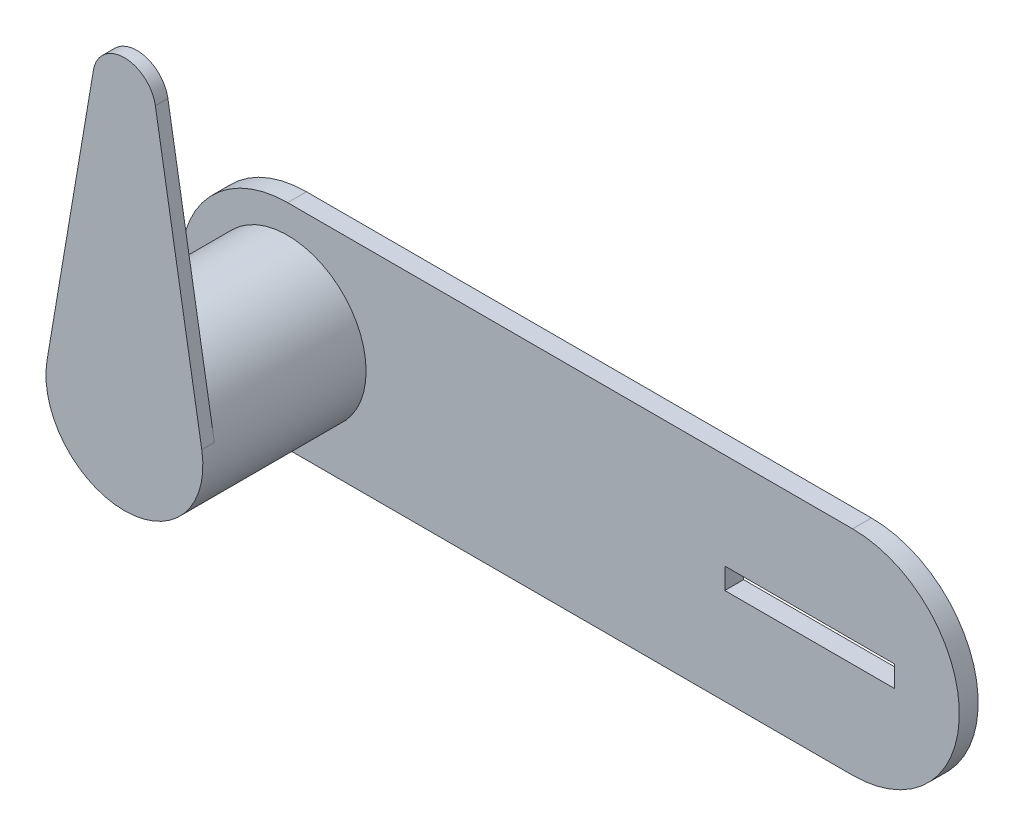
from build123d import *

# Parameters (mm, degrees)
EXTRUDE_1_DEPTH     = 3
SKETCH_2_W          = 27.052742461
SKETCH_2_H          = 3.381592808
CUT_EXTRUDE_1_DEPTH = 3
SKETCH_3_R          = 12.5
EXTRUDE_2_DEPTH     = 24
EXTRUDE_3_DEPTH     = 2


with BuildPart() as part:
    # 草图1 → 凸台-拉伸1 (new body)
    with BuildSketch(Plane.XY):
        with BuildLine():
            Line((-45, 17), (45, 17))
            ThreePointArc((45, 17), (62, 0), (45, -17))
            Line((45, -17), (-45, -17))
            ThreePointArc((-45, -17), (-62, 0), (-45, 17))
        make_face()
    extrude(amount=EXTRUDE_1_DEPTH)

    # 草图2 → 切除-拉伸1 (cut)
    with BuildSketch(Plane(origin=(0, 0, 0), x_dir=(-1, 0, 0), z_dir=(0, 0, -1))):
        with Locations((-38.163690258, 0)):
            Rectangle(SKETCH_2_W, SKETCH_2_H)
    extrude(amount=-CUT_EXTRUDE_1_DEPTH, mode=Mode.SUBTRACT)

    # 草图3 → 凸台-拉伸2 (add)
    with BuildSketch(Plane.XY.offset(3)):
        with Locations((-45, 0)):
            Circle(SKETCH_3_R)
    extrude(amount=EXTRUDE_2_DEPTH)

    # 草图4 → 凸台-拉伸3 (add)
    with BuildSketch(Plane.XY.offset(27)):
        with BuildLine():
            Line((-57.325166215, 2.083333333), (-49.930066486, 45.833333333))
            ThreePointArc((-49.930066486, 45.833333333), (-45, 50), (-40.069933514, 45.833333333))
            Line((-40.069933514, 45.833333333), (-32.674833785, 2.083333333))
            ThreePointArc((-32.674833785, 2.083333333), (-45, -12.5), (-57.325166215, 2.083333333))
        make_face()
    extrude(amount=EXTRUDE_3_DEPTH)


solid = part.part
